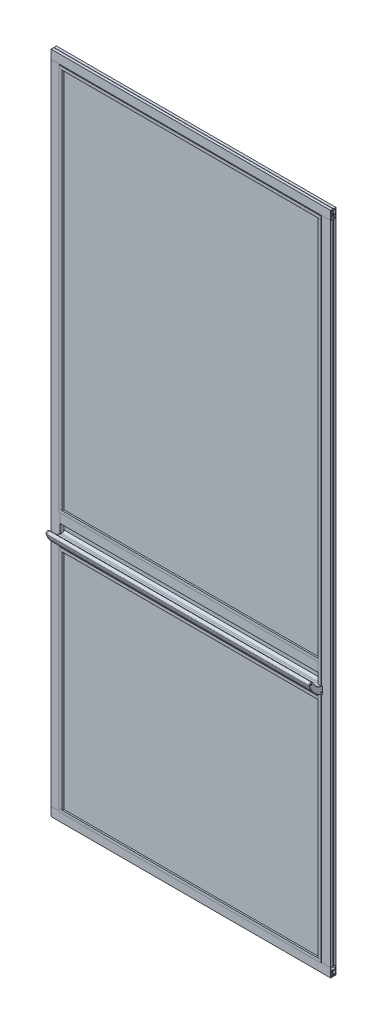
from build123d import *

# Parameters (mm, degrees)
D_XXXXXX_XX_XXXX_XXXX_XXXXXX_XXX_XXXXXXX_DEPTH = 940
D_XXXXXX_XX_XXXX_XXXX_XXXXXX_XXX_XXX_2_DEPTH   = 940
D_XXXXXX_XX_XXXX_XXXX_XXXXXX_XXX_XXX_3_DEPTH   = 2238
D_XXXXXX_XX_XXXX_XXXX_XXXXXX_XXX_XXX_5_DEPTH   = 2238
EXTRUDE_2705_DEPTH                             = 880
EXTRUDE_2952_DEPTH                             = 880
EXTRUDE_START                                  = 10
EXTRUDE_3223_DEPTH                             = 2156
EXTRUDE_3223_2_DEPTH                           = 2156
SKETCH_2_W                                     = 872
SKETCH_2_H                                     = 2168
EXTRUDE_3851_DEPTH                             = 17
SKETCH_17_W                                    = 856
SKETCH_17_H                                    = 2152
EXTRUDE_10_DEPTH                               = 6
EXTRUDE_2_DEPTH                                = 880
SKETCH_6_R                                     = 2
EXTRUDE_3_DEPTH                                = 3
SKETCH_7_R                                     = 2
EXTRUDE_4_DEPTH                                = 2
SKETCH_8_R                                     = 2
EXTRUDE_5_DEPTH                                = 3
CUT_EXTRUDE_4_DEPTH                            = 1443.516115394
CUT_EXTRUDE_4_DEPTH_BACK                       = 1443.516115394
SKETCH_14_W                                    = 30
SKETCH_14_H                                    = 120
CUT_EXTRUDE_5_DEPTH                            = 1443.516115394
CUT_EXTRUDE_5_DEPTH_BACK                       = 1443.516115394
SKETCH_15_W                                    = 19.3
SKETCH_15_H                                    = 108
CUT_EXTRUDE_6_DEPTH                            = 1435.976216936
CUT_EXTRUDE_6_DEPTH_BACK                       = 1435.976216936
SKETCH_18_W                                    = 6
SKETCH_18_H                                    = 124


with BuildPart() as part:
    # Sketch1 → D_xxxxxx_xx_xxxx_xxxx_xxxxxx_xxx_xxxxxxx (new body)
    with BuildSketch(Plane(origin=(-470, 1118, 0), x_dir=(0, 0, -1), z_dir=(1, 0, 0))):
        with BuildLine():
            Line((-0.5, 0), (-9, 0))
            Line((-9, 0), (-9, -30))
            Line((-9, -30), (-5.9, -30))
            Line((-5.9, -30), (-5.9, -28.5))
            Line((-5.9, -28.5), (-7, -28.5))
            Line((-7, -28.5), (-7, -20))
            Line((-7, -20), (7, -20))
            Line((7, -20), (7, -28.5))
            Line((7, -28.5), (5.9, -28.5))
            Line((5.9, -28.5), (5.9, -30))
            Line((5.9, -30), (9, -30))
            Line((9, -30), (9, 0))
            Line((9, 0), (0.5, 0))
            ThreePointArc((0.5, 0), (0, -0.5), (-0.5, 0))
        make_face()
        with BuildLine():
            Line((-1.341640787, -3), (1.341640786, -3))
            ThreePointArc((1.341640786, -3), (1.799302724, -4.250096987), (1.272792206, -5.472792206))
            ThreePointArc((1.272792206, -5.472792206), (1.272792206, -6.250609665), (2.050609665, -6.250609665))
            ThreePointArc((2.050609665, -6.250609665), (2.853462499, -4.717447359), (2.640075756, -3))
            Line((2.640075756, -3), (7, -3))
            Line((7, -3), (7, -18))
            Line((7, -18), (2.640075756, -18))
            ThreePointArc((2.640075756, -18), (2.853462499, -16.282552641), (2.050609665, -14.749390335))
            ThreePointArc((2.050609665, -14.749390335), (1.272792206, -14.749390335), (1.272792206, -15.527207794))
            ThreePointArc((1.272792206, -15.527207794), (1.799302724, -16.749903013), (1.341640786, -18))
            Line((1.341640786, -18), (-1.341640787, -18))
            ThreePointArc((-1.341640787, -18), (-1.799302724, -16.749903013), (-1.272792206, -15.527207794))
            ThreePointArc((-1.272792206, -15.527207794), (-1.272792206, -14.749390335), (-2.050609665, -14.749390335))
            ThreePointArc((-2.050609665, -14.749390335), (-2.853462499, -16.282552641), (-2.640075756, -18))
            Line((-2.640075756, -18), (-7, -18))
            Line((-7, -18), (-7, -3))
            Line((-7, -3), (-2.640075756, -3))
            ThreePointArc((-2.640075756, -3), (-2.853462499, -4.717447359), (-2.050609665, -6.250609665))
            ThreePointArc((-2.050609665, -6.250609665), (-1.272792206, -6.250609665), (-1.272792206, -5.472792206))
            ThreePointArc((-1.272792206, -5.472792206), (-1.799302724, -4.250096987), (-1.341640787, -3))
        make_face(mode=Mode.SUBTRACT)
    extrude(amount=D_XXXXXX_XX_XXXX_XXXX_XXXXXX_XXX_XXXXXXX_DEPTH)


with BuildPart() as body_2:
    # Sketch1 on segment 2 (carried to segment 2) → D_xxxxxx_xx_xxxx_xxxx_xxxxxx_xxx_xxx 2 (new body)
    with BuildSketch(Plane(origin=(-470, -1118, 0), x_dir=(0, 0, 1), z_dir=(1, 0, 0))):
        with BuildLine():
            Line((-0.5, 0), (-9, 0))
            Line((-9, 0), (-9, -30))
            Line((-9, -30), (-5.9, -30))
            Line((-5.9, -30), (-5.9, -28.5))
            Line((-5.9, -28.5), (-7, -28.5))
            Line((-7, -28.5), (-7, -20))
            Line((-7, -20), (7, -20))
            Line((7, -20), (7, -28.5))
            Line((7, -28.5), (5.9, -28.5))
            Line((5.9, -28.5), (5.9, -30))
            Line((5.9, -30), (9, -30))
            Line((9, -30), (9, 0))
            Line((9, 0), (0.5, 0))
            ThreePointArc((0.5, 0), (0, -0.5), (-0.5, 0))
        make_face()
        with BuildLine():
            Line((-1.341640787, -3), (1.341640786, -3))
            ThreePointArc((1.341640786, -3), (1.799302724, -4.250096987), (1.272792206, -5.472792206))
            ThreePointArc((1.272792206, -5.472792206), (1.272792206, -6.250609665), (2.050609665, -6.250609665))
            ThreePointArc((2.050609665, -6.250609665), (2.853462499, -4.717447359), (2.640075756, -3))
            Line((2.640075756, -3), (7, -3))
            Line((7, -3), (7, -18))
            Line((7, -18), (2.640075756, -18))
            ThreePointArc((2.640075756, -18), (2.853462499, -16.282552641), (2.050609665, -14.749390335))
            ThreePointArc((2.050609665, -14.749390335), (1.272792206, -14.749390335), (1.272792206, -15.527207794))
            ThreePointArc((1.272792206, -15.527207794), (1.799302724, -16.749903013), (1.341640786, -18))
            Line((1.341640786, -18), (-1.341640787, -18))
            ThreePointArc((-1.341640787, -18), (-1.799302724, -16.749903013), (-1.272792206, -15.527207794))
            ThreePointArc((-1.272792206, -15.527207794), (-1.272792206, -14.749390335), (-2.050609665, -14.749390335))
            ThreePointArc((-2.050609665, -14.749390335), (-2.853462499, -16.282552641), (-2.640075756, -18))
            Line((-2.640075756, -18), (-7, -18))
            Line((-7, -18), (-7, -3))
            Line((-7, -3), (-2.640075756, -3))
            ThreePointArc((-2.640075756, -3), (-2.853462499, -4.717447359), (-2.050609665, -6.250609665))
            ThreePointArc((-2.050609665, -6.250609665), (-1.272792206, -6.250609665), (-1.272792206, -5.472792206))
            ThreePointArc((-1.272792206, -5.472792206), (-1.799302724, -4.250096987), (-1.341640787, -3))
        make_face(mode=Mode.SUBTRACT)
    extrude(amount=D_XXXXXX_XX_XXXX_XXXX_XXXXXX_XXX_XXX_2_DEPTH)


with BuildPart() as body_3:
    # Sketch1 on segment 3 (carried to segment 3) → D_xxxxxx_xx_xxxx_xxxx_xxxxxx_xxx_xxx 3 (new body)
    with BuildSketch(Plane(origin=(470, 1119, 0), x_dir=(0, 0, -1), z_dir=(0, -1, 0))):
        with BuildLine():
            Line((-0.5, 0), (-9, 0))
            Line((-9, 0), (-9, -30))
            Line((-9, -30), (-5.9, -30))
            Line((-5.9, -30), (-5.9, -28.5))
            Line((-5.9, -28.5), (-7, -28.5))
            Line((-7, -28.5), (-7, -20))
            Line((-7, -20), (7, -20))
            Line((7, -20), (7, -28.5))
            Line((7, -28.5), (5.9, -28.5))
            Line((5.9, -28.5), (5.9, -30))
            Line((5.9, -30), (9, -30))
            Line((9, -30), (9, 0))
            Line((9, 0), (0.5, 0))
            ThreePointArc((0.5, 0), (0, -0.5), (-0.5, 0))
        make_face()
        with BuildLine():
            Line((-1.341640787, -3), (1.341640786, -3))
            ThreePointArc((1.341640786, -3), (1.799302724, -4.250096987), (1.272792206, -5.472792206))
            ThreePointArc((1.272792206, -5.472792206), (1.272792206, -6.250609665), (2.050609665, -6.250609665))
            ThreePointArc((2.050609665, -6.250609665), (2.853462499, -4.717447359), (2.640075756, -3))
            Line((2.640075756, -3), (7, -3))
            Line((7, -3), (7, -18))
            Line((7, -18), (2.640075756, -18))
            ThreePointArc((2.640075756, -18), (2.853462499, -16.282552641), (2.050609665, -14.749390335))
            ThreePointArc((2.050609665, -14.749390335), (1.272792206, -14.749390335), (1.272792206, -15.527207794))
            ThreePointArc((1.272792206, -15.527207794), (1.799302724, -16.749903013), (1.341640786, -18))
            Line((1.341640786, -18), (-1.341640787, -18))
            ThreePointArc((-1.341640787, -18), (-1.799302724, -16.749903013), (-1.272792206, -15.527207794))
            ThreePointArc((-1.272792206, -15.527207794), (-1.272792206, -14.749390335), (-2.050609665, -14.749390335))
            ThreePointArc((-2.050609665, -14.749390335), (-2.853462499, -16.282552641), (-2.640075756, -18))
            Line((-2.640075756, -18), (-7, -18))
            Line((-7, -18), (-7, -3))
            Line((-7, -3), (-2.640075756, -3))
            ThreePointArc((-2.640075756, -3), (-2.853462499, -4.717447359), (-2.050609665, -6.250609665))
            ThreePointArc((-2.050609665, -6.250609665), (-1.272792206, -6.250609665), (-1.272792206, -5.472792206))
            ThreePointArc((-1.272792206, -5.472792206), (-1.799302724, -4.250096987), (-1.341640787, -3))
        make_face(mode=Mode.SUBTRACT)
    extrude(amount=D_XXXXXX_XX_XXXX_XXXX_XXXXXX_XXX_XXX_3_DEPTH)

    # D_xxxxxx_xx_xxxx_xxxx_xxxxxx_xxx_xxx 3 e
    split(bisect_by=Plane(origin=(470, 1088, 0), x_dir=(1, 0, 0), z_dir=(0, -1, 0)), keep=Keep.TOP)

    # D_xxxxxx_xx_xxxx_xxxx_xxxxxx_xxx_xxx 4
    split(bisect_by=Plane(origin=(470, -1088, 0), x_dir=(-1, 0, 0), z_dir=(0, 1, 0)), keep=Keep.TOP)


with BuildPart() as body_4:
    # Sketch1 on segment 4 (carried to segment 4) → D_xxxxxx_xx_xxxx_xxxx_xxxxxx_xxx_xxx 5 (new body)
    with BuildSketch(Plane(origin=(-470, 1119, 0), x_dir=(0, 0, 1), z_dir=(0, -1, 0))):
        with BuildLine():
            Line((-0.5, 0), (-9, 0))
            Line((-9, 0), (-9, -30))
            Line((-9, -30), (-5.9, -30))
            Line((-5.9, -30), (-5.9, -28.5))
            Line((-5.9, -28.5), (-7, -28.5))
            Line((-7, -28.5), (-7, -20))
            Line((-7, -20), (7, -20))
            Line((7, -20), (7, -28.5))
            Line((7, -28.5), (5.9, -28.5))
            Line((5.9, -28.5), (5.9, -30))
            Line((5.9, -30), (9, -30))
            Line((9, -30), (9, 0))
            Line((9, 0), (0.5, 0))
            ThreePointArc((0.5, 0), (0, -0.5), (-0.5, 0))
        make_face()
        with BuildLine():
            Line((-1.341640787, -3), (1.341640786, -3))
            ThreePointArc((1.341640786, -3), (1.799302724, -4.250096987), (1.272792206, -5.472792206))
            ThreePointArc((1.272792206, -5.472792206), (1.272792206, -6.250609665), (2.050609665, -6.250609665))
            ThreePointArc((2.050609665, -6.250609665), (2.853462499, -4.717447359), (2.640075756, -3))
            Line((2.640075756, -3), (7, -3))
            Line((7, -3), (7, -18))
            Line((7, -18), (2.640075756, -18))
            ThreePointArc((2.640075756, -18), (2.853462499, -16.282552641), (2.050609665, -14.749390335))
            ThreePointArc((2.050609665, -14.749390335), (1.272792206, -14.749390335), (1.272792206, -15.527207794))
            ThreePointArc((1.272792206, -15.527207794), (1.799302724, -16.749903013), (1.341640786, -18))
            Line((1.341640786, -18), (-1.341640787, -18))
            ThreePointArc((-1.341640787, -18), (-1.799302724, -16.749903013), (-1.272792206, -15.527207794))
            ThreePointArc((-1.272792206, -15.527207794), (-1.272792206, -14.749390335), (-2.050609665, -14.749390335))
            ThreePointArc((-2.050609665, -14.749390335), (-2.853462499, -16.282552641), (-2.640075756, -18))
            Line((-2.640075756, -18), (-7, -18))
            Line((-7, -18), (-7, -3))
            Line((-7, -3), (-2.640075756, -3))
            ThreePointArc((-2.640075756, -3), (-2.853462499, -4.717447359), (-2.050609665, -6.250609665))
            ThreePointArc((-2.050609665, -6.250609665), (-1.272792206, -6.250609665), (-1.272792206, -5.472792206))
            ThreePointArc((-1.272792206, -5.472792206), (-1.799302724, -4.250096987), (-1.341640787, -3))
        make_face(mode=Mode.SUBTRACT)
    extrude(amount=D_XXXXXX_XX_XXXX_XXXX_XXXXXX_XXX_XXX_5_DEPTH)

    # D_xxxxxx_xx_xxxx_xxxx_xxxxxx_xxx_xxx 5 e
    split(bisect_by=Plane(origin=(-470, 1088, 0), x_dir=(1, 0, 0), z_dir=(0, -1, 0)), keep=Keep.TOP)

    # D_xxxxxx_xx_xxxx_xxxx_xxxxxx_xxx_xxx 6
    split(bisect_by=Plane(origin=(-470, -1088, 0), x_dir=(-1, 0, 0), z_dir=(0, 1, 0)), keep=Keep.TOP)


with BuildPart() as body_5:
    # 草图10 → Extrude 2705 (new body)
    with BuildSketch(Plane(origin=(-440, 0, 0), x_dir=(0, 0, -1), z_dir=(1, 0, 0))):
        Polygon((12.7, 1086), (12.7, 1078), (18.2, 1078), (18.2, 1088), (6, 1088), (6, 1096), (4.2, 1096), (4.2, 1088.000000001), (-4.1, 1088), (-4.1, 1096), (-5.9, 1096), (-5.9, 1088), (-11.8, 1088), (-11.8, 1078), (-6.6, 1078), (-6.6, 1086), align=None)
    extrude(amount=EXTRUDE_2705_DEPTH)


with BuildPart() as body_6:
    # 草图11 → Extrude 2952 (new body)
    with BuildSketch(Plane(origin=(-440, 0, 0), x_dir=(0, 0, -1), z_dir=(1, 0, 0))):
        Polygon((12.7, -1086), (12.7, -1078), (18.2, -1078), (18.2, -1088), (6, -1088), (6, -1096), (4.2, -1096), (4.2, -1088.000000001), (-4.1, -1088), (-4.1, -1096), (-5.9, -1096), (-5.9, -1088), (-11.8, -1088), (-11.8, -1078), (-6.6, -1078), (-6.6, -1086), align=None)
    extrude(amount=EXTRUDE_2952_DEPTH)


with BuildPart() as body_7:
    # 草图12 → Extrude 3223 (new body)
    with BuildSketch(Plane(origin=(0, -1088, 0), x_dir=(1, 0, 0), z_dir=(0, 1, 0)).offset(EXTRUDE_START)):
        Polygon((-438, 12.7), (-430, 12.7), (-430, 18.2), (-440, 18.2), (-440, 6), (-448, 6), (-448, 4.2), (-440.000000001, 4.2), (-440, -4.1), (-448, -4.1), (-448, -5.9), (-440, -5.9), (-440, -11.8), (-430, -11.8), (-430, -6.6), (-438, -6.6), align=None)
    extrude(amount=EXTRUDE_3223_DEPTH)

    # 草图14 → 切除-拉伸4 (cut, two sides: drawn at the far end of the back side and taken through both)
    with BuildSketch(Plane.ZY.offset(440).offset(-CUT_EXTRUDE_4_DEPTH_BACK)):
        with Locations((-3.2, -265)):
            Rectangle(SKETCH_14_W, SKETCH_14_H)
    extrude(amount=CUT_EXTRUDE_4_DEPTH + CUT_EXTRUDE_4_DEPTH_BACK, mode=Mode.SUBTRACT)


with BuildPart() as body_8:
    # 草图12 → Extrude 3223 2 (new body)
    with BuildSketch(Plane(origin=(0, -1088, 0), x_dir=(1, 0, 0), z_dir=(0, 1, 0)).offset(EXTRUDE_START)):
        Polygon((438, 12.7), (430, 12.7), (430, 18.2), (440, 18.2), (440, 6), (448, 6), (448, 4.2), (440.000000001, 4.2), (440, -4.1), (448, -4.1), (448, -5.9), (440, -5.9), (440, -11.8), (430, -11.8), (430, -6.6), (438, -6.6), align=None)
    extrude(amount=EXTRUDE_3223_2_DEPTH)


with BuildPart() as body_9:
    # 草图2 → Extrude 3851 (new body)
    with BuildSketch(Plane.XY.offset(6.6)):
        Rectangle(SKETCH_2_W, SKETCH_2_H)
    extrude(amount=-EXTRUDE_3851_DEPTH)

    # 草图15 → 切除-拉伸5 (cut, two sides: drawn at the far end of the back side and taken through both)
    with BuildSketch(Plane.ZY.offset(440).offset(-CUT_EXTRUDE_5_DEPTH_BACK)):
        with Locations((-3.05, -265)):
            Rectangle(SKETCH_15_W, SKETCH_15_H)
    extrude(amount=CUT_EXTRUDE_5_DEPTH + CUT_EXTRUDE_5_DEPTH_BACK, mode=Mode.SUBTRACT)


with BuildPart() as body_10:
    # 草图17 → 凸台-拉伸10 (new body)
    with BuildSketch(Plane(origin=(0, 0, -10.4), x_dir=(-1, 0, 0), z_dir=(0, 0, -1))):
        Rectangle(SKETCH_17_W, SKETCH_17_H)
    extrude(amount=EXTRUDE_10_DEPTH)

    # 草图18 → 切除-拉伸6 (cut, two sides: drawn at the far end of the back side and taken through both)
    with BuildSketch(Plane.ZY.offset(428).offset(-CUT_EXTRUDE_6_DEPTH_BACK)):
        with Locations((-13.4, -265)):
            Rectangle(SKETCH_18_W, SKETCH_18_H)
    extrude(amount=CUT_EXTRUDE_6_DEPTH + CUT_EXTRUDE_6_DEPTH_BACK, mode=Mode.SUBTRACT)


with BuildPart() as body_11:
    # 草图4 → 凸台-拉伸2 (new body)
    with BuildSketch(Plane.ZY.offset(-440)):
        with BuildLine():
            Line((2.857553645, -247.108927406), (6.704462631, -245.385112329))
            ThreePointArc((6.704462631, -245.385112329), (6.919661361, -245.200645134), (7, -244.928828391))
            Line((7, -244.928828391), (7, -242.952423581))
            ThreePointArc((7, -242.952423581), (6.121320344, -240.831103238), (4, -239.952423581))
            Line((4, -239.952423581), (-4, -239.952423581))
            ThreePointArc((-4, -239.952423581), (-4.707106781, -240.2453168), (-5, -240.952423581))
            Line((-5, -240.952423581), (-5, -249.086015321))
            ThreePointArc((-5, -249.086015321), (-4.543633488, -249.925338042), (-3.591074738, -249.998583198))
            Line((-3.591074738, -249.998583198), (-3.347907918, -249.889619187))
            ThreePointArc((-3.347907918, -249.889619187), (-3.194897044, -249.885245411), (-3.08360929, -249.99034771))
            Line((-3.08360929, -249.99034771), (-2.895538614, -250.410050952))
            ThreePointArc((-2.895538614, -250.410050952), (-2.8816414, -250.529556054), (-2.938818386, -250.635411588))
            Line((-2.938818386, -250.635411588), (-3.678508693, -251.352733376))
            Line((-3.678508693, -251.352733376), (-3.596723641, -251.535246951))
            Line((-3.596723641, -251.535246951), (-3.140439702, -251.33078432))
            ThreePointArc((-3.140439702, -251.33078432), (-2.941801607, -251.350985338), (-2.859622684, -251.532951814))
            Line((-2.859622684, -251.532951814), (-3.131422947, -254.285427902))
            Line((-3.131422947, -254.285427902), (-5, -255.122744643))
            Line((-5, -255.122744643), (-5, -274.876431855))
            ThreePointArc((-5, -274.876431855), (-1.310885546, -278.990696117), (4, -280.517532911))
            Line((4, -280.517532911), (9, -280.517532911))
            ThreePointArc((9, -280.517532911), (29.001605349, -272.801616047), (41.658705692, -255.498512265))
            ThreePointArc((41.658705692, -255.498512265), (49.190680956, -252.177818295), (52.949400099, -259.50104779))
            ThreePointArc((52.949400099, -259.50104779), (36.94100116, -286.960097621), (10.522889115, -304.633569556))
            Line((10.522889115, -304.633569556), (9, -304.633569556))
            Line((9, -304.633569556), (9, -315))
            Line((9, -315), (5.9, -315))
            Line((5.9, -315), (5.9, -313.5))
            Line((5.9, -313.5), (7, -313.5))
            Line((7, -313.5), (7, -305))
            Line((7, -305), (-7, -305))
            Line((-7, -305), (-7, -313.5))
            Line((-7, -313.5), (-5.9, -313.5))
            Line((-5.9, -313.5), (-5.9, -315))
            Line((-5.9, -315), (-9, -315))
            Line((-9, -315), (-9, -305))
            Line((-9, -305), (-8.5, -304.5))
            Line((-8.5, -304.5), (-8.5, -302.5))
            Line((-8.5, -302.5), (-9, -302))
            Line((-9, -302), (-9, -228))
            Line((-9, -228), (-8.5, -227.5))
            Line((-8.5, -227.5), (-8.5, -225.5))
            Line((-8.5, -225.5), (-9, -225))
            Line((-9, -225), (-9, -215))
            Line((-9, -215), (-5.9, -215))
            Line((-5.9, -215), (-5.9, -216.5))
            Line((-5.9, -216.5), (-7, -216.5))
            Line((-7, -216.5), (-7, -225))
            Line((-7, -225), (7, -225))
            Line((7, -225), (7, -216.5))
            Line((7, -216.5), (5.9, -216.5))
            Line((5.9, -216.5), (5.9, -215))
            Line((5.9, -215), (9, -215))
            Line((9, -215), (9, -248.849289471))
            Line((9, -248.849289471), (6.9068237, -249.78725002))
            Line((6.9068237, -249.78725002), (5.994255823, -250.196175282))
            Line((5.994255823, -250.196175282), (3.759062035, -248.567093108))
            ThreePointArc((3.759062035, -248.567093108), (3.677947451, -248.384649697), (3.795076163, -248.222952329))
            Line((3.795076163, -248.222952329), (4.251360101, -248.018489698))
            Line((4.251360101, -248.018489698), (4.169575049, -247.835976122))
            Line((4.169575049, -247.835976122), (3.141897681, -247.910618755))
            ThreePointArc((3.141897681, -247.910618755), (3.024838296, -247.882839225), (2.944895799, -247.792929275))
            Line((2.944895799, -247.792929275), (2.756825122, -247.373226034))
            ThreePointArc((2.756825122, -247.373226034), (2.752451346, -247.220215159), (2.857553645, -247.108927406))
        make_face()
        with BuildLine():
            Line((-0.591607978, -302), (0.591607978, -302))
            ThreePointArc((0.591607978, -302), (1.754528537, -300.702031856), (1.272792206, -299.027207794))
            ThreePointArc((1.272792206, -299.027207794), (1.272792206, -298.249390335), (2.050609665, -298.249390335))
            ThreePointArc((2.050609665, -298.249390335), (2.8908371, -300.069650561), (2.349468025, -302))
            Line((2.349468025, -302), (7, -302))
            Line((7, -302), (7, -282.517532911))
            Line((7, -282.517532911), (4, -282.517532911))
            ThreePointArc((4, -282.517532911), (-1.098439293, -281.380585741), (-5.230769231, -278.185185708))
            ThreePointArc((-5.230769231, -278.185185708), (-6.33968311, -277.883616831), (-7, -278.824156774))
            Line((-7, -278.824156774), (-7, -302))
            Line((-7, -302), (-2.349468025, -302))
            ThreePointArc((-2.349468025, -302), (-2.890837099, -300.069650561), (-2.050609666, -298.249390335))
            ThreePointArc((-2.050609666, -298.249390335), (-1.272792206, -298.249390335), (-1.272792206, -299.027207794))
            ThreePointArc((-1.272792206, -299.027207794), (-1.754528537, -300.702031855), (-0.591607978, -302))
        make_face(mode=Mode.SUBTRACT)
        with BuildLine():
            Line((-2.349468025, -228), (-7, -228))
            Line((-7, -228), (-7, -237.952423581))
            Line((-7, -237.952423581), (7, -237.952423581))
            Line((7, -237.952423581), (7, -228))
            Line((7, -228), (2.349468025, -228))
            ThreePointArc((2.349468025, -228), (2.890837099, -229.930349439), (2.050609665, -231.750609665))
            ThreePointArc((2.050609665, -231.750609665), (1.272792206, -231.750609665), (1.272792206, -230.972792206))
            ThreePointArc((1.272792206, -230.972792206), (1.754528537, -229.297968144), (0.591607978, -228))
            Line((0.591607978, -228), (-0.591607978, -228))
            ThreePointArc((-0.591607978, -228), (-1.754528537, -229.297968144), (-1.272792206, -230.972792206))
            ThreePointArc((-1.272792206, -230.972792206), (-1.272792206, -231.750609665), (-2.050609665, -231.750609665))
            ThreePointArc((-2.050609665, -231.750609665), (-2.8908371, -229.930349439), (-2.349468025, -228))
        make_face(mode=Mode.SUBTRACT)
        with BuildLine():
            Line((47.990278547, -260.512974914), (49.42470127, -260.93826723))
            ThreePointArc((49.42470127, -260.93826723), (49.72344908, -261.181787003), (49.760223756, -261.565453207))
            ThreePointArc((49.760223756, -261.565453207), (37.064728814, -284.546306856), (16.273739662, -300.57846193))
            ThreePointArc((16.273739662, -300.57846193), (15.889893701, -300.600604766), (15.603815834, -300.34372448))
            Line((15.603815834, -300.34372448), (14.904952734, -298.876313524))
            ThreePointArc((14.904952734, -298.876313524), (16.389996434, -297.529474766), (16.646469065, -295.541120868))
            ThreePointArc((16.646469065, -295.541120868), (15.98776331, -295.127470377), (15.574112819, -295.786176132))
            ThreePointArc((15.574112819, -295.786176132), (12.86209147, -297.711531202), (13.418348531, -294.432410889))
            ThreePointArc((13.418348531, -294.432410889), (13.831999022, -293.773705134), (13.173293267, -293.360054644))
            ThreePointArc((13.173293267, -293.360054644), (11.493703581, -294.45472716), (10.925592049, -296.377376042))
            Line((10.925592049, -296.377376042), (9.5, -296.377376042))
            ThreePointArc((9.5, -296.377376042), (9.146446609, -296.230929432), (9, -295.877376042))
            Line((9, -295.877376042), (9, -282.025929779))
            ThreePointArc((9, -282.025929779), (28.875214056, -274.716759873), (42.854511276, -258.809926508))
            ThreePointArc((42.854511276, -258.809926508), (43.15129036, -258.559946567), (43.537497896, -258.597516964))
            Line((43.537497896, -258.597516964), (44.790550315, -259.274708837))
            ThreePointArc((44.790550315, -259.274708837), (45.415980474, -259.180714504), (45.539471562, -258.560434108))
            ThreePointArc((45.539471562, -258.560434108), (47.83577205, -256.154388388), (47.913373649, -259.479449279))
            ThreePointArc((47.913373649, -259.479449279), (47.587164388, -260.023346665), (47.990278547, -260.512974914))
        make_face(mode=Mode.SUBTRACT)
    extrude(amount=EXTRUDE_2_DEPTH)


with BuildPart() as body_12:
    # 草图6 → 凸台-拉伸3 (new body)
    with BuildSketch(Plane.ZY.offset(440)):
        with BuildLine():
            Line((9.5, -304.633569556), (10.522889115, -304.633569556))
            ThreePointArc((10.522889115, -304.633569556), (36.94100116, -286.960097621), (52.949400099, -259.50104779))
            ThreePointArc((52.949400099, -259.50104779), (49.190680956, -252.177818295), (41.658705691, -255.498512265))
            ThreePointArc((41.658705691, -255.498512265), (29.200353014, -272.648317686), (9.5, -280.472796488))
            Line((9.5, -280.472796488), (9.5, -304.633569556))
        make_face()
        with Locations((47.185930191, -257.832990651)):
            Circle(SKETCH_6_R, mode=Mode.SUBTRACT)
        with Locations((13.819348054, -296.187175655)):
            Circle(SKETCH_6_R, mode=Mode.SUBTRACT)
    extrude(amount=EXTRUDE_3_DEPTH)


with BuildPart() as body_13:
    # 草图7 → 凸台-拉伸4 (new body)
    with BuildSketch(Plane.ZY.offset(440)):
        Polygon((-5.7, -228), (-5.7, -239.952423581), (-3.7, -239.952423581), (-3.7, -249.952423581), (-5.7, -249.952423581), (-5.7, -302), (-3.7, -304), (3.7, -304), (5.7, -302), (5.7, -249.952423581), (3.7, -249.952423581), (3.7, -239.952423581), (5.7, -239.952423581), (5.7, -228), (3.7, -226), (-3.7, -226), align=None)
        with Locations((0, -229.7)):
            Circle(SKETCH_7_R, mode=Mode.SUBTRACT)
        with Locations((0, -300.3)):
            Circle(SKETCH_7_R, mode=Mode.SUBTRACT)
    extrude(amount=EXTRUDE_4_DEPTH)


with BuildPart() as body_14:
    # 草图8 → 凸台-拉伸5 (new body)
    with BuildSketch(Plane.ZY.offset(442)):
        Polygon((-6.7, -228), (-6.7, -239.952423581), (-3.7, -239.952423581), (-3.7, -249.952423581), (-6.7, -249.952423581), (-6.7, -302), (-4.7, -304), (4.7, -304), (6.7, -302), (6.7, -249.952423581), (3.7, -249.952423581), (3.7, -239.952423581), (6.7, -239.952423581), (6.7, -228), (4.7, -226), (-4.7, -226), align=None)
        with Locations((0, -229.7)):
            Circle(SKETCH_8_R, mode=Mode.SUBTRACT)
        with Locations((0, -300.3)):
            Circle(SKETCH_8_R, mode=Mode.SUBTRACT)
    extrude(amount=EXTRUDE_5_DEPTH)


with BuildPart() as body_15:
    # 镜向1: mirrored copy
    add(body_12.part.mirror(Plane(origin=(0, 0, 0), x_dir=(0, 0, 1), z_dir=(1, 0, 0))))


with BuildPart() as body_16:
    # Mirror 1 2: mirrored copy
    add(body_13.part.mirror(Plane(origin=(0, 0, 0), x_dir=(0, 0, 1), z_dir=(1, 0, 0))))


with BuildPart() as body_17:
    # Mirror 1 3: mirrored copy
    add(body_14.part.mirror(Plane(origin=(0, 0, 0), x_dir=(0, 0, 1), z_dir=(1, 0, 0))))


with BuildPart() as body_18:
    # 镜向2: mirrored copy
    add(body_5.part.mirror(Plane(origin=(0, 436.5, 0), x_dir=(0, 0, 1), z_dir=(0, -1, 0))))


with BuildPart() as body_19:
    # 镜向3: mirrored copy
    add(body_6.part.mirror(Plane(origin=(0, -701.5, 0), x_dir=(0, 0, 1), z_dir=(0, -1, 0))))


with BuildPart() as cut_extrude_4_piece_1:
    # of the separate pieces the step leaves, piece 1, a body of its own (cut_extrude_4_pieces)
    add(body_7.part.solids().sort_by_distance((-438, -205, -12.7))[0])


with BuildPart() as cut_extrude_4_piece_2:
    # of the separate pieces the step leaves, piece 2, a body of its own (cut_extrude_4_pieces)
    add(body_7.part.solids().sort_by_distance((-438, -1078, -12.7))[0])


with BuildPart() as cut_extrude_5_piece_1:
    # of the separate pieces the step leaves, piece 1, a body of its own (cut_extrude_5_pieces)
    add(body_9.part.solids().sort_by_distance((-436, 1084, 6.6))[0])


with BuildPart() as cut_extrude_5_piece_2:
    # of the separate pieces the step leaves, piece 2, a body of its own (cut_extrude_5_pieces)
    add(body_9.part.solids().sort_by_distance((-436, -1084, 6.6))[0])


with BuildPart() as cut_extrude_6_piece_1:
    # of the separate pieces the step leaves, piece 1, a body of its own (cut_extrude_6_pieces)
    add(body_10.part.solids().sort_by_distance((428, 1076, -10.4))[0])


with BuildPart() as cut_extrude_6_piece_2:
    # of the separate pieces the step leaves, piece 2, a body of its own (cut_extrude_6_pieces)
    add(body_10.part.solids().sort_by_distance((428, -1076, -10.4))[0])


solid = Compound([part.part, body_2.part, body_3.part, body_4.part, body_5.part, body_6.part, body_8.part, body_11.part, body_12.part, body_13.part, body_14.part, body_15.part, body_16.part, body_17.part, body_18.part, body_19.part, cut_extrude_4_piece_1.part, cut_extrude_4_piece_2.part, cut_extrude_5_piece_1.part, cut_extrude_5_piece_2.part, cut_extrude_6_piece_1.part, cut_extrude_6_piece_2.part])
